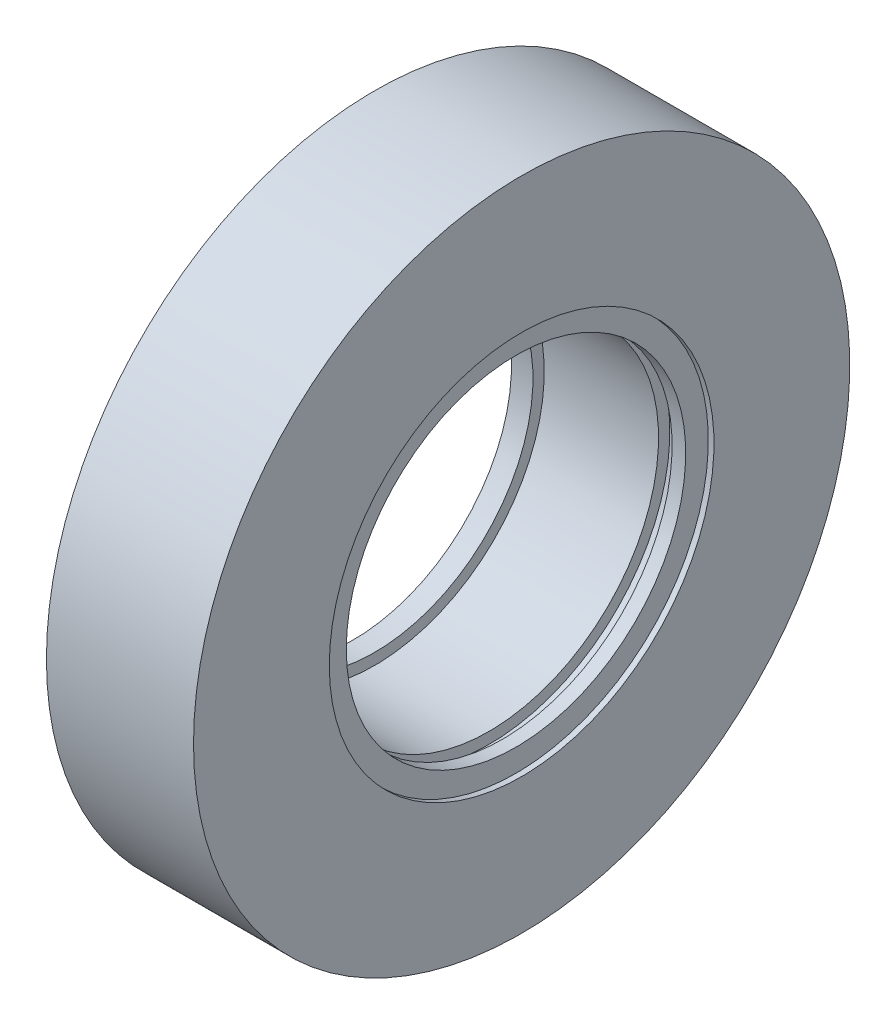
from build123d import *


with BuildPart() as part:
    # 草图2 → 旋转1 (revolve)
    with BuildSketch(Plane.XY, mode=Mode.PRIVATE) as revolve_1_sk:
        Polygon((0, 14), (1.9, 14), (1.9, 15), (12, 15), (12, 16), (13.2, 16), (13.2, 15), (14.4, 15), (14.4, 17), (14.9, 17), (14.9, 29), (1.9, 29), (1.9, 25), (0, 25), align=None)
    revolve(revolve_1_sk.sketch.rotate(Axis((-10.496116508, 0, 0), (1, 0, 0)), 90), axis=Axis((-10.496116508, 0, 0), (1, 0, 0)))


solid = part.part
